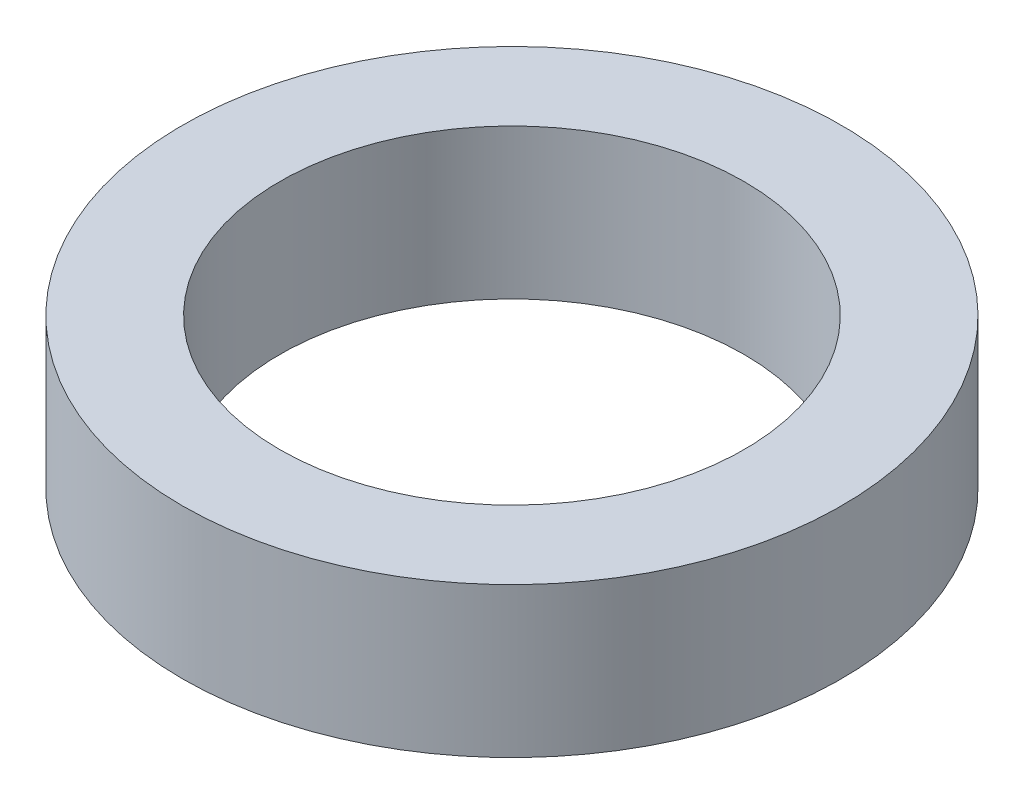
SolidWorks part; units mm, degrees
ref_plane "Front Plane" through (0, 0, 0) normal (0, 0, 1) x (1, 0, 0)
ref_plane "Top Plane" through (0, 0, 0) normal (0, 1, 0) x (1, 0, 0)
ref_plane "Right Plane" through (0, 0, 0) normal (1, 0, 0) x (0, 0, -1)
other "Configuration Table"
sketch "Sketch2" plane through (0, 0, 0) normal (0, 1, 0) x (1, 0, 0)
  circle A0 centre (0, 0) radius 11
  dimension "D1" = 22
extrude "Boss-Extrude1" add sketch "Sketch2" along normal blind 5
hole_wizard "M18 Tapped Hole1" positions "Sketch5" profile "Sketch4" tap size "M18" standard "GB" end condition up to next
sketch "Sketch5" plane through (0, 5, 0) normal (0, 1, 0) x (1, 0, 0)
  point P0 (0, 0)
sketch "Sketch4" plane through (0, 5, 0) normal (1, 0, 0) x (0, 0, 1)
  line L0 (0, 0) -> (0, 5)
  line L1 (0, 5) -> (7.75, 5)
  line L2 (7.75, 5) -> (7.75, 0)
  line L5 (7.75, 0) -> (0, 0)
  line L11 (0, -6.35) -> (0, 107.95) construction
  dimension "通孔螺纹孔钻头直径" = 15.5
  dimension "通孔螺纹孔钻头深度" = 5
cosmetic thread "Cosmetic Thread 1"
